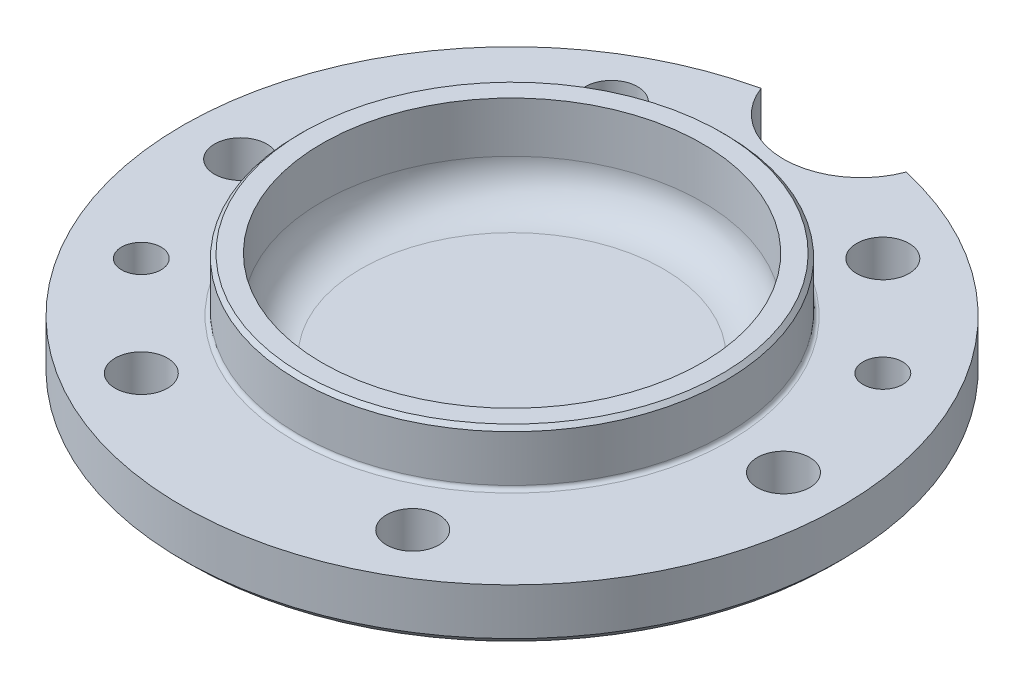
from build123d import *

# Parameters (mm, degrees)
SKETCH1_R           = 85
BOSS_EXTRUDE1_DEPTH = 14
SKETCH2_R           = 55
BOSS_EXTRUDE2_DEPTH = 14
SKETCH3_R           = 49
CUT_EXTRUDE1_DEPTH  = 23
FILLET1_R           = 10
FILLET2_R           = 1
CHAMFER1_SIZE       = 1
SKETCH4_R           = 20
SKETCH4_R_2         = 6.75
CUT_EXTRUDE2_DEPTH  = 122.020659393
M12_TAPPED_HOLE1_D  = 10.2
CHAMFER2_SIZE       = 2


with BuildPart() as part:
    # Sketch1 → Boss-Extrude1 (new body)
    with BuildSketch(Plane(origin=(0, 0, 0), x_dir=(1, 0, 0), z_dir=(0, 1, 0))):
        with Locations(Location((0, 0, 0), (0, 0, 270))):
            Circle(SKETCH1_R)
    extrude(amount=BOSS_EXTRUDE1_DEPTH)

    # Sketch2 → Boss-Extrude2 (add)
    with BuildSketch(Plane(origin=(0, 14, 0), x_dir=(1, 0, 0), z_dir=(0, 1, 0))):
        with Locations(Location((0, 0, 0), (0, 0, 270))):
            Circle(SKETCH2_R)
    extrude(amount=BOSS_EXTRUDE2_DEPTH)

    # Sketch3 → Cut-Extrude1 (cut)
    with BuildSketch(Plane(origin=(0, 28, 0), x_dir=(1, 0, 0), z_dir=(0, 1, 0))):
        with Locations(Location((0, 0, 0), (0, 0, 270))):
            Circle(SKETCH3_R)
    extrude(amount=-CUT_EXTRUDE1_DEPTH, mode=Mode.SUBTRACT)

    # Fillet1
    fillet1_edges = [part.edges().sort_by_distance(p)[0] for p in [
        (0, 5, -49),
    ]]
    fillet(fillet1_edges, radius=FILLET1_R)

    # Fillet2
    fillet2_edges = [part.edges().sort_by_distance(p)[0] for p in [
        (0, 14, -55),
    ]]
    fillet(fillet2_edges, radius=FILLET2_R)

    # Chamfer1
    chamfer1_edges = [part.edges().sort_by_distance(p)[0] for p in [
        (0, 28, -55),
    ]]
    chamfer(chamfer1_edges, length=CHAMFER1_SIZE)

    # Sketch4 → Cut-Extrude2 (cut, through all)
    with BuildSketch(Plane(origin=(0, 14, 0), x_dir=(1, 0, 0), z_dir=(0, 1, 0))):
        with Locations((0, 90)):
            Circle(SKETCH4_R)
        with Locations(Location((-35, 60.621778265, 0), (0, 0, 270))):
            Circle(SKETCH4_R_2)
        with Locations(Location((35, 60.621778265, 0), (0, 0, 270))):
            Circle(SKETCH4_R_2)
        with Locations(Location((70, 0, 0), (0, 0, 270))):
            Circle(SKETCH4_R_2)
        with Locations(Location((35, -60.621778265, 0), (0, 0, 270))):
            Circle(SKETCH4_R_2)
        with Locations(Location((-35, -60.621778265, 0), (0, 0, 270))):
            Circle(SKETCH4_R_2)
        with Locations(Location((-70, 0, 0), (0, 0, 270))):
            Circle(SKETCH4_R_2)
    extrude(amount=-CUT_EXTRUDE2_DEPTH, mode=Mode.SUBTRACT)

    # M12 Tapped Hole1 (through all)
    with Locations(Plane(origin=(0, 14, 0), x_dir=(1, 0, 0), z_dir=(0, 1, 0))):
        with Locations((-60.621778265, -35), (60.621778265, 35)):
            Hole(M12_TAPPED_HOLE1_D / 2)

    # Chamfer2
    chamfer2_edges = [part.edges().sort_by_distance(p)[0] for p in [
        (0, 0, 85),
        (0, 0, -70),
    ]]
    chamfer(chamfer2_edges, length=CHAMFER2_SIZE)


solid = part.part
